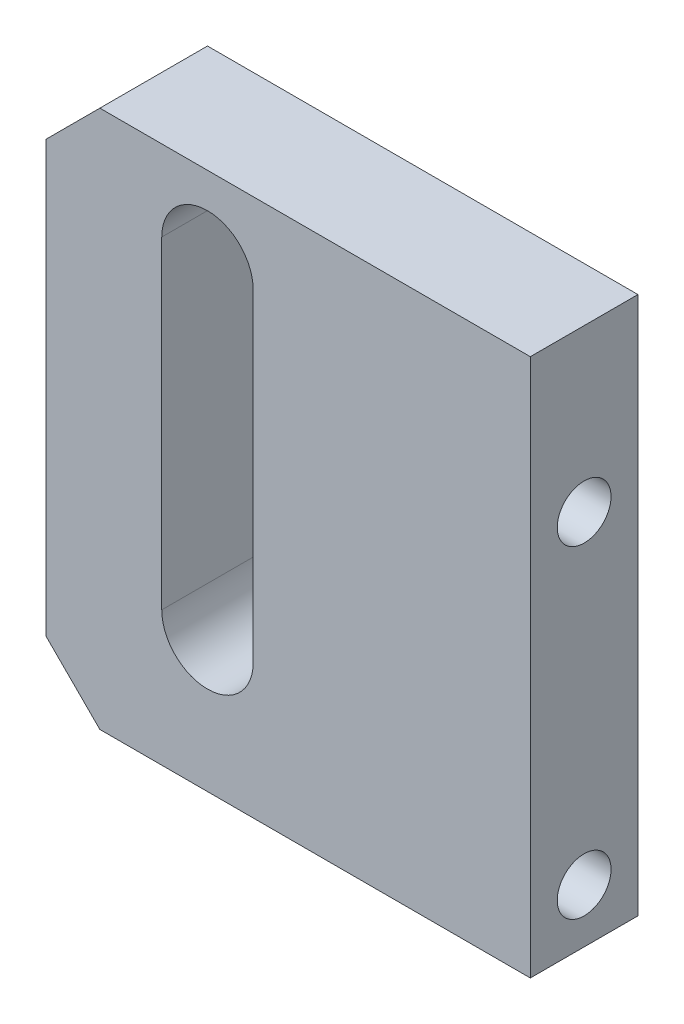
SolidWorks part; units mm, degrees
ref_plane "Front Plane" through (0, 0, 0) normal (0, 0, 1) x (1, 0, 0)
ref_plane "Top Plane" through (0, 0, 0) normal (0, 1, 0) x (1, 0, 0)
ref_plane "Right Plane" through (0, 0, 0) normal (1, 0, 0) x (0, 0, -1)
sketch "Sketch1" plane through (0, 0, 0) normal (0, 0, 1) x (1, 0, 0)
  line L1 (-32.787, 47.8421) -> (12.213, 47.8421)
  line L2 (-32.787, 47.8421) -> (-32.787, -2.1579)
  line L3 (-32.787, -2.1579) -> (12.213, -2.1579)
  line L4 (12.213, 47.8421) -> (12.213, -2.1579)
  dimension "D1" = 45
  dimension "D2" = 50
extrude "Boss-Extrude1" add sketch "Sketch1" along normal blind 10
sketch "Sketch2" plane through (0, 0, 10) normal (0, 0, 1) x (1, 0, 0)
  line L0 (-17.787, 40.3421) -> (-17.787, 10.3421) construction
  line L1 (-13.537, 40.3421) -> (-13.537, 10.3421)
  line L2 (-22.037, 40.3421) -> (-22.037, 10.3421)
  line L3 (12.213, -2.1579) -> (12.213, 47.8421) construction
  line L5 (12.213, 47.8421) -> (-32.787, 47.8421) construction
  arc A0 (-13.537, 40.3421) -> (-22.037, 40.3421) centre (-17.787, 40.3421) ccw
  arc A1 (-22.037, 10.3421) -> (-13.537, 10.3421) centre (-17.787, 10.3421) ccw
  point P2 (-17.787, 25.3421)
  dimension "D1" = 8.5
  dimension "D2" = 30
  dimension "D3" = 7.5
  dimension "D4" = 30
  dimension "D5" = 30
extrude "Cut-Extrude1" cut sketch "Sketch2" against normal through all
chamfer "Chamfer1" distance 5 angle 45 2 edges at (-32.787, 47.8421, 5) (-32.787, -2.1579, 5)
hole_wizard "M6 Tapped Hole1" positions "Sketch3" profile "Sketch4" tap size "M6" standard "ISO"
sketch "Sketch3" plane through (12.213, 0, 0) normal (1, 0, 0) x (0, 0, -1)
  line L0 (-5, 47.8421) -> (-5, -8.1916) construction
  line L1 (-10, 47.8421) -> (0, 47.8421) construction
  line L3 (-10, -2.1579) -> (0, -2.1579) construction
  point P0 (-5, 32.8421)
  point P2 (-5, 2.8421)
  dimension "D1" = 30
  dimension "D2" = 5
sketch "Sketch4" plane through (12.213, 32.8421, 5) normal (0, 1, 0) x (0, 0, -1)
  line L0 (0, 0) -> (0, 20.5022)
  line L1 (0, 20.5022) -> (2.5, 19)
  line L2 (2.5, 19) -> (2.5, 0)
  line L5 (2.5, 0) -> (0, 0)
  line L10 (0, 20.5022) -> (-2.5, 19) construction
  line L11 (0, -6.35) -> (0, 107.95) construction
  dimension "螺纹孔钻头直径" = 5
  dimension "螺纹孔钻头深度" = 19
  dimension "导头角度" = 118
cosmetic thread "Cosmetic thread1" parameters "D1"=16, "D2"=6
cosmetic thread "Cosmetic thread2" parameters "D1"=16, "D2"=6
